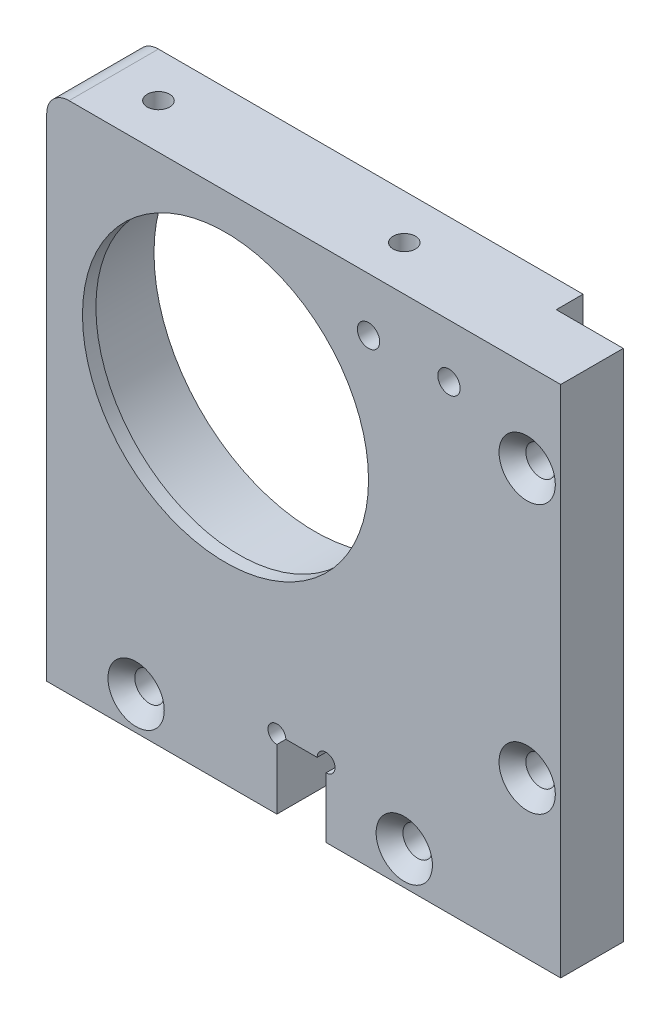
SolidWorks part; units mm, degrees
ref_plane "前视基准面" through (0, 0, 0) normal (0, 0, 1) x (1, 0, 0)
ref_plane "上视基准面" through (0, 0, 0) normal (0, 1, 0) x (1, 0, 0)
ref_plane "右视基准面" through (0, 0, 0) normal (1, 0, 0) x (0, 0, -1)
sketch "草图1" plane through (0, 0, 0) normal (0, 0, 1) x (1, 0, 0)
  line L1 (-57.5, 57.5) -> (57.5, 57.5)
  line L2 (-57.5, 57.5) -> (-57.5, -57.5)
  line L3 (-57.5, -57.5) -> (57.5, -57.5)
  line L4 (57.5, 57.5) -> (57.5, -57.5)
  line L5 (-57.5, 57.5) -> (57.5, -57.5) construction
  line L6 (-57.5, -57.5) -> (57.5, 57.5) construction
  point P0 (0, 0)
  dimension "D1" = 115
  dimension "D2" = 115
extrude "凸台-拉伸1" add sketch "草图1" along normal blind 20
sketch "草图2" plane through (0, 0, 0) normal (0, 0, -1) x (-1, 0, 0)
  line L0 (-57.5, 57.5) -> (-42.5, 57.5)
  line L1 (-57.5, 57.5) -> (57.5, 57.5) construction
  line L2 (-42.5, 57.5) -> (-42.5, -42.5)
  line L3 (-42.5, -42.5) -> (57.5, -42.5)
  line L4 (57.5, 57.5) -> (57.5, -57.5) construction
  line L5 (57.5, -42.5) -> (57.5, -57.5)
  line L6 (57.5, -57.5) -> (-57.5, -57.5)
  line L7 (-57.5, -57.5) -> (-57.5, 57.5)
  dimension "D1" = 15
extrude "切除-拉伸1" cut sketch "草图2" against normal blind 6
sketch "草图3" plane through (0, 0, 0) normal (0, 0, -1) x (-1, 0, 0)
  line L0 (-42.5, 57.5) -> (57.5, 57.5) construction
  line L1 (57.5, 57.5) -> (57.5, -42.5) construction
  circle A0 centre (17.5, 17.5) radius 32
  dimension "D1" = 64
  dimension "D2" = 40
  dimension "D3" = 40
extrude "切除-拉伸2" cut sketch "草图3" against normal through all
sketch "草图4" plane through (0, 0, 0) normal (0, 0, -1) x (-1, 0, 0)
  circle A0 centre (17.5, 17.5) radius 36
  dimension "D1" = 72
extrude "切除-拉伸3" cut sketch "草图4" against normal blind 17
sketch "草图5" plane through (0, 0, 20) normal (0, 0, 1) x (1, 0, 0)
  line L0 (-57.5, 57.5) -> (-57.5, -57.5) construction
  line L1 (-6, -57.5) -> (5, -57.5)
  line L2 (-6, -57.5) -> (-6, -42)
  line L3 (-6, -42) -> (5, -42)
  line L4 (5, -57.5) -> (5, -42)
  line L5 (-57.5, -57.5) -> (57.5, -57.5) construction
  dimension "D1" = 51.5
  dimension "D2" = 11
  dimension "D3" = 15.5
extrude "切除-拉伸4" cut sketch "草图5" against normal through all
sketch "草图6" plane through (0, 0, 20) normal (0, 0, 1) x (1, 0, 0)
  circle A0 centre (-6, -42) radius 2
  circle A1 centre (5, -42) radius 2
  dimension "D1" = 4
extrude "切除-拉伸5" cut sketch "草图6" against normal through all
hole_wizard "M6 锥坑平头螺钉的锥形沉头孔1" positions "草图7" profile "草图8" countersink size "M6" standard "ISO" end condition through all
sketch "草图7" plane through (0, 0, 20) normal (0, 0, 1) x (1, 0, 0)
  line L0 (-57.5, 57.5) -> (-57.5, -57.5) construction
  line L1 (-57.5, -57.5) -> (-6, -57.5) construction
  line L2 (-37.5, -50) -> (22.5, -50) construction
  line L3 (22.5, -50) -> (50, -50) construction
  line L4 (50, -50) -> (50, 51.4478) construction
  line L5 (57.5, -57.5) -> (57.5, 57.5) construction
  line L6 (57.5, 57.5) -> (-57.5, 57.5) construction
  point P0 (-37.5, -50)
  point P2 (22.5, -50)
  point P4 (50, -22.5)
  point P6 (50, 37.5)
  dimension "D1" = 20
  dimension "D2" = 60
  dimension "D3" = 7.5
  dimension "D4" = 7.5
  dimension "D5" = 20
  dimension "D6" = 60
sketch "草图8" plane through (-37.5, -50, 20) normal (1, 0, 0) x (0, -1, 0)
  line L0 (0, 0) -> (0, 20)
  line L1 (0, 20) -> (3.3, 20)
  line L2 (3.3, 20) -> (3.3, 3)
  line L3 (3.3, 3) -> (6.3, 0)
  line L5 (6.3, 0) -> (0, 0)
  line L6 (-3.3, 3) -> (-6.3, 0) construction
  line L11 (0, -6.35) -> (0, 107.95) construction
  dimension "通孔孔直径" = 6.6
  dimension "通孔孔深度" = 20
  dimension "近端锥形沉头孔直径" = 12.6
  dimension "近端锥形沉头孔角度" = 90
fillet "圆角1" radius 5 1 edges at (-57.5, 57.5, 10)
hole_wizard "M6 螺纹孔1" positions "草图9" profile "草图10" tap size "M6" standard "GB"
sketch "草图9" plane through (0, 0, 20) normal (0, 0, 1) x (1, 0, 0)
  line L0 (14.5, 45.5) -> (32.5, 45.5) construction
  line L2 (57.5, 57.5) -> (-52.5, 57.5) construction
  line L3 (57.5, -57.5) -> (57.5, 57.5) construction
  point P0 (32.5, 45.5)
  point P2 (14.5, 45.5)
  dimension "D1" = 12
  dimension "D2" = 25
  dimension "D3" = 18
cosmetic thread "孔螺蚊线1" parameters "D1"=12, "D2"=6
cosmetic thread "孔螺蚊线2" parameters "D1"=12, "D2"=6
sketch "草图10" plane through (32.5, 45.5, 20) normal (1, 0, 0) x (0, -1, 0)
  line L0 (0, 0) -> (0, 18.5022)
  line L1 (0, 18.5022) -> (2.5, 17)
  line L2 (2.5, 17) -> (2.5, 0)
  line L5 (2.5, 0) -> (0, 0)
  line L10 (0, 18.5022) -> (-2.5, 17) construction
  line L11 (0, -6.35) -> (0, 107.95) construction
  dimension "螺纹孔钻头直径" = 5
  dimension "螺纹孔钻头深度" = 17
  dimension "导头角度" = 118
hole_wizard "M6 螺纹孔2" positions "草图11" profile "草图12" tap size "M6" standard "GB"
sketch "草图11" plane through (0, 57.5, 0) normal (0, 1, 0) x (1, 0, 0)
  line L0 (-57.5, -10) -> (-42.5, -10) construction
  line L1 (-57.5, -20) -> (-57.5, 0) construction
  line L3 (-42.5, -10) -> (12.5, -10) construction
  point P0 (-42.5, -10)
  point P16 (12.5, -10)
  dimension "D1" = 15
  dimension "D2" = 55
sketch "草图12" plane through (-42.5, 57.5, 10) normal (1, 0, 0) x (0, 0, 1)
  line L0 (0, 0) -> (0, 18.5022)
  line L1 (0, 18.5022) -> (2.5, 17)
  line L2 (2.5, 17) -> (2.5, 0)
  line L5 (2.5, 0) -> (0, 0)
  line L10 (0, 18.5022) -> (-2.5, 17) construction
  line L11 (0, -6.35) -> (0, 107.95) construction
  dimension "螺纹孔钻头直径" = 5
  dimension "螺纹孔钻头深度" = 17
  dimension "导头角度" = 118
cosmetic thread "孔螺蚊线3" parameters "D1"=12, "D2"=6
cosmetic thread "孔螺蚊线4" parameters "D1"=12, "D2"=6
